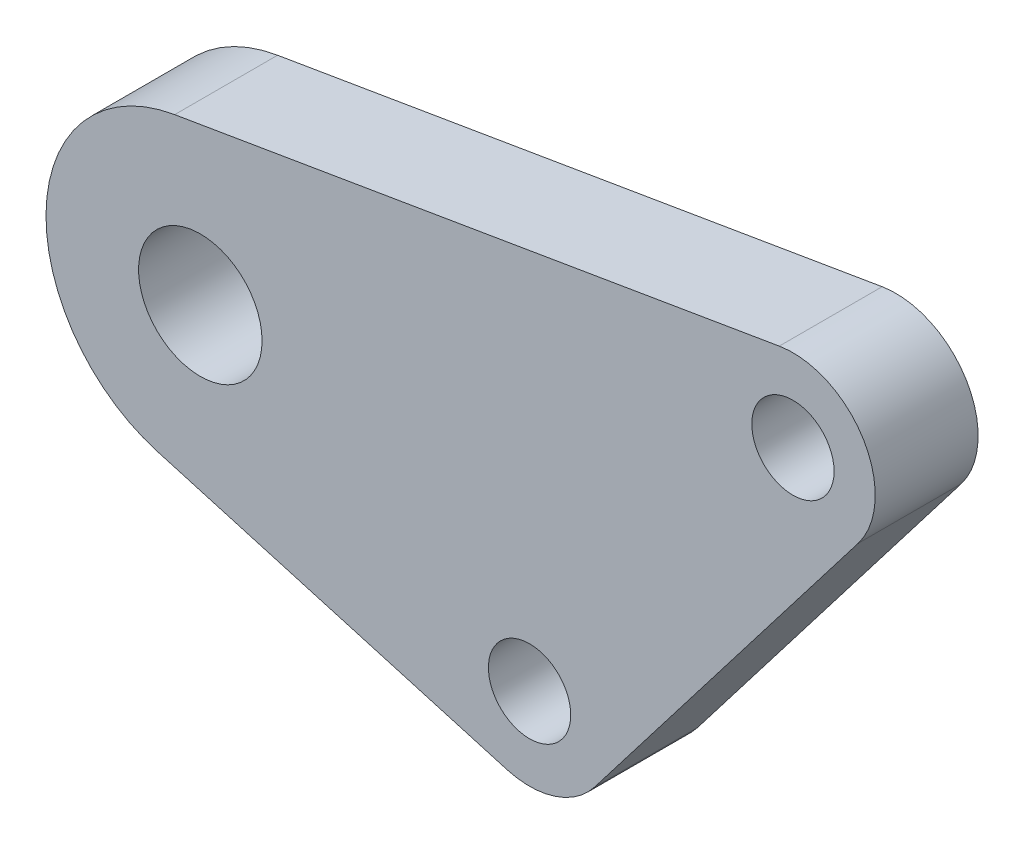
from build123d import *

# Parameters (mm, degrees)
SKETCH1_R           = 2
SKETCH1_R_2         = 3
BOSS_EXTRUDE1_DEPTH = 5


with BuildPart() as part:
    # Sketch1 → Boss-Extrude1 (new body)
    with BuildSketch(Plane.XY):
        with BuildLine():
            Line((-17.245659368, 15.645832119), (12.135648337, 20.594443797))
            ThreePointArc((12.135648337, 20.594443797), (16.228516711, 18.710406067), (15.971203863, 14.212077511))
            Line((15.971203863, 14.212077511), (3.171203863, -2.437922489))
            ThreePointArc((3.171203863, -2.437922489), (1.248757853, -3.80007945), (-1.106950177, -3.843782162))
            Line((-1.106950177, -3.843782162), (-18.075531582, 1.042908447))
            ThreePointArc((-18.075531582, 1.042908447), (-23.487918421, 8.675532282), (-17.245659368, 15.645832119))
        make_face()
        Circle(SKETCH1_R, mode=Mode.SUBTRACT)
        with Locations((-16, 8.25)):
            Circle(SKETCH1_R_2, mode=Mode.SUBTRACT)
        with Locations((12.8, 16.65)):
            Circle(SKETCH1_R, mode=Mode.SUBTRACT)
    extrude(amount=BOSS_EXTRUDE1_DEPTH)


solid = part.part
